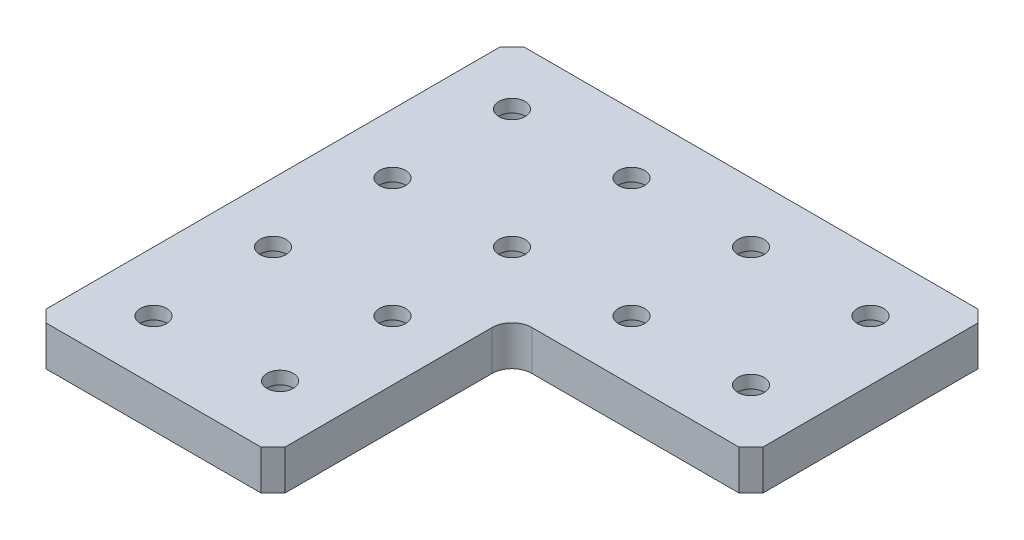
from build123d import *

# Parameters (mm, degrees)
SKETCH_1_W                = 120
SKETCH_1_H                = 120
EXTRUDE_1_DEPTH           = 10
SKETCH_2_W                = 60
SKETCH_2_H                = 60
CUT_EXTRUDE_1_DEPTH       = 25
CHAMFER_1_SIZE            = 3
FILLET_1_R                = 5
HOLE_WIZARD_1_D           = 6.6
HOLE_WIZARD_1_DEPTH       = 25
HOLE_WIZARD_1_CBORE_D     = 11
HOLE_WIZARD_1_CBORE_DEPTH = 6.8
HOLE_WIZARD_1_TIP         = 1.982840043


with BuildPart() as part:
    # 草图1 → 凸台-拉伸1 (new body)
    with BuildSketch(Plane(origin=(0, 0, 0), x_dir=(1, 0, 0), z_dir=(0, 1, 0))):
        Rectangle(SKETCH_1_W, SKETCH_1_H)
    extrude(amount=EXTRUDE_1_DEPTH)

    # 草图2 → 切除-拉伸1 (cut)
    with BuildSketch(Plane(origin=(0, 10, 0), x_dir=(1, 0, 0), z_dir=(0, 1, 0))):
        with Locations((30, -30)):
            Rectangle(SKETCH_2_W, SKETCH_2_H)
    extrude(amount=-CUT_EXTRUDE_1_DEPTH, mode=Mode.SUBTRACT)

    # 倒角1
    chamfer_1_edges = [part.edges().sort_by_distance(p)[0] for p in [
        (60, 5, 0),
        (0, 5, 60),
        (-60, 5, 60),
        (-60, 5, -60),
        (60, 5, -60),
    ]]
    chamfer(chamfer_1_edges, length=CHAMFER_1_SIZE)

    # 圆角1
    fillet_1_edges = [part.edges().sort_by_distance(p)[0] for p in [
        (0, 5, 0),
    ]]
    fillet(fillet_1_edges, radius=FILLET_1_R)

    # 打孔尺寸(%根据)内六角圆柱头螺钉的类型1
    with Locations(Plane(origin=(0, 0, 0), x_dir=(-1, 0, 0), z_dir=(0, -1, 0))):
        with Locations((45, 45), (45, 15), (15, 45), (15, 15), (-45, 45), (-45, 15), (45, -15), (45, -45), (15, -43.223897071), (15, -15), (-15, 45), (-15, 15)):
            CounterBoreHole(HOLE_WIZARD_1_D / 2, HOLE_WIZARD_1_CBORE_D / 2, HOLE_WIZARD_1_CBORE_DEPTH, depth=HOLE_WIZARD_1_DEPTH)
            with Locations((0, 0, -(HOLE_WIZARD_1_DEPTH + HOLE_WIZARD_1_TIP / 2))):  # 118° drill point
                Cone(0, HOLE_WIZARD_1_D / 2, HOLE_WIZARD_1_TIP, mode=Mode.SUBTRACT)


solid = part.part
